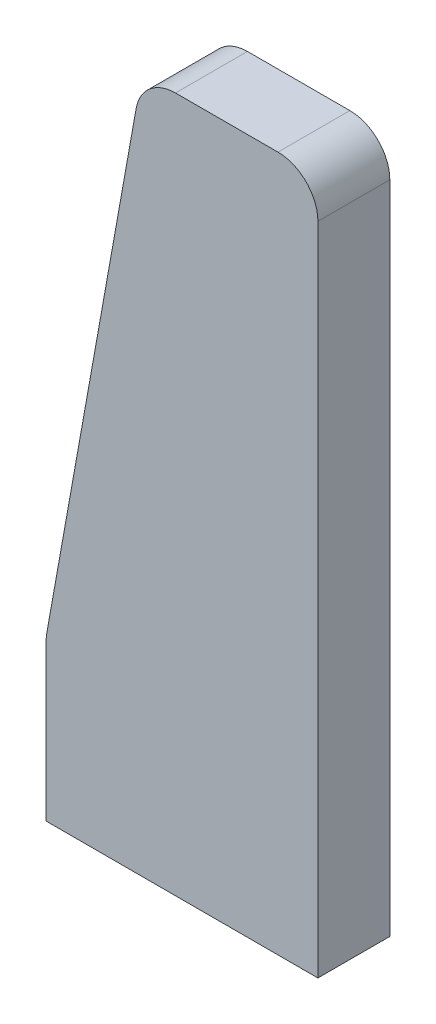
SolidWorks part; units mm, degrees
ref_plane "Front Plane" through (0, 0, 0) normal (0, 0, 1) x (1, 0, 0)
ref_plane "Top Plane" through (0, 0, 0) normal (0, 1, 0) x (1, 0, 0)
ref_plane "Right Plane" through (0, 0, 0) normal (1, 0, 0) x (0, 0, -1)
sketch "Sketch1" plane through (0, 0, 0) normal (0, 0, 1) x (1, 0, 0)
  line L0 (0, 0) -> (-34, 0)
  line L1 (-34, 0) -> (-34, 19.5558)
  line L2 (0, 0) -> (0, 82)
  line L3 (-5, 87) -> (-17.816, 87)
  line L4 (-33.9217, 20.4373) -> (-22.7376, 82.8815)
  arc A0 (0, 82) -> (-5, 87) centre (-5, 82) ccw
  arc A1 (-34, 19.5558) -> (-33.9217, 20.4373) centre (-29, 19.5558) cw
  arc A2 (-17.816, 87) -> (-22.7376, 82.8815) centre (-17.816, 82) ccw
  dimension "D1" = 5
extrude "Boss-Extrude1" add sketch "Sketch1" along normal blind 9
